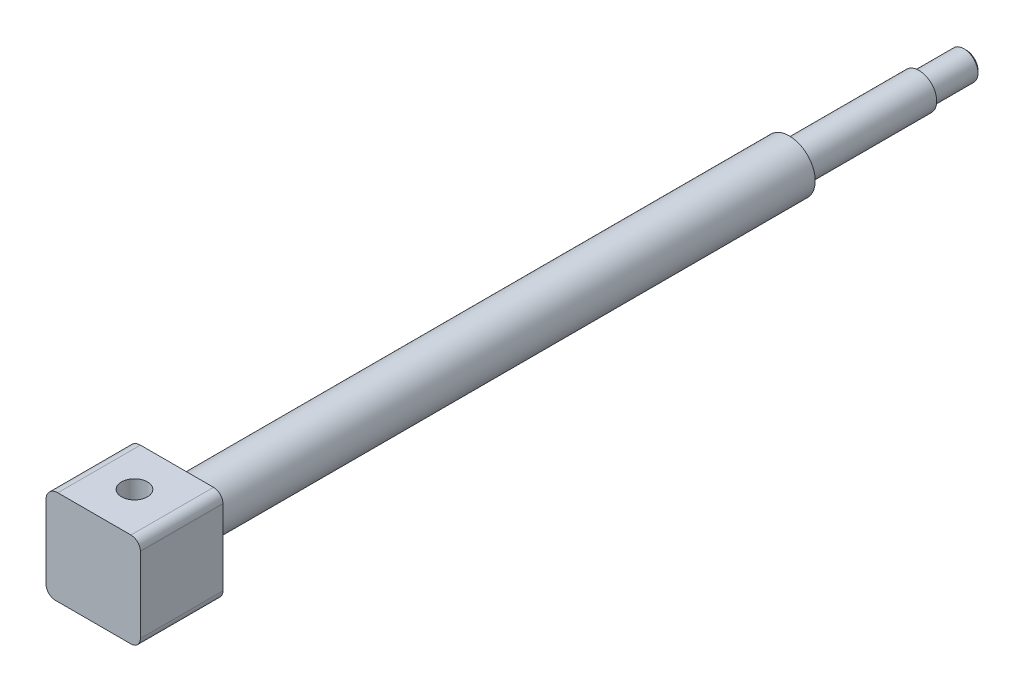
SolidWorks part; units mm, degrees
ref_plane "Front Plane" through (0, 0, 0) normal (0, 0, 1) x (1, 0, 0)
ref_plane "Top Plane" through (0, 0, 0) normal (0, 1, 0) x (1, 0, 0)
ref_plane "Right Plane" through (0, 0, 0) normal (1, 0, 0) x (0, 0, -1)
sketch "Sketch1" plane through (0, 0, 0) normal (0, 0, 1) x (1, 0, 0)
  line L1 (-15, 20) -> (16.0113, 20)
  line L2 (-20, 15) -> (-20, -16.0113)
  line L3 (-16.0113, -20) -> (16.0113, -20)
  line L4 (20, 16.0113) -> (20, -16.0113)
  line L5 (-20, 20) -> (20, -20) construction
  line L6 (-20, -20) -> (20, 20) construction
  arc A0 (-20, 15) -> (-15, 20) centre (-15, 15) cw
  arc A1 (-16.0113, -20) -> (-20, -16.0113) centre (-16.0113, -16.0113) cw
  arc A2 (16.0113, -20) -> (20, -16.0113) centre (16.0113, -16.0113) ccw
  arc A3 (20, 16.0113) -> (16.0113, 20) centre (16.0113, 16.0113) ccw
  point P0 (0, 0)
  dimension "D3" = 5
  dimension "D4" = 3.9887
  dimension "D1" = 40
  dimension "D2" = 40
extrude "Boss-Extrude2" add sketch "Sketch1" along normal mid plane 35
sketch "Sketch3" plane through (0, 20, 0) normal (0, 1, 0) x (1, 0, 0)
  circle A0 centre (0, 0) radius 5.5
  dimension "D1" = 11
extrude "Cut-Extrude2" cut sketch "Sketch3" against normal blind 54
sketch "Sketch4" plane through (0, 0, -17.5) normal (0, 0, -1) x (-1, 0, 0)
  circle A0 centre (0, 0) radius 11
  dimension "D1" = 22
extrude "Boss-Extrude3" add sketch "Sketch4" along normal blind 260
sketch "Sketch5" plane through (0, 0, -277.5) normal (0, 0, -1) x (-1, 0, 0)
  circle A0 centre (0, 0) radius 7.5
  dimension "D1" = 15
extrude "Boss-Extrude4" add sketch "Sketch5" along normal blind 55
sketch "Sketch6" plane through (0, 0, -332.5) normal (0, 0, -1) x (-1, 0, 0)
  circle A0 centre (0, 0) radius 6
  dimension "D1" = 12
extrude "Boss-Extrude5" add sketch "Sketch6" along normal blind 20
chamfer "Chamfer1" distance 1 angle 45 1 edges at (-6, 0, -352.5)
